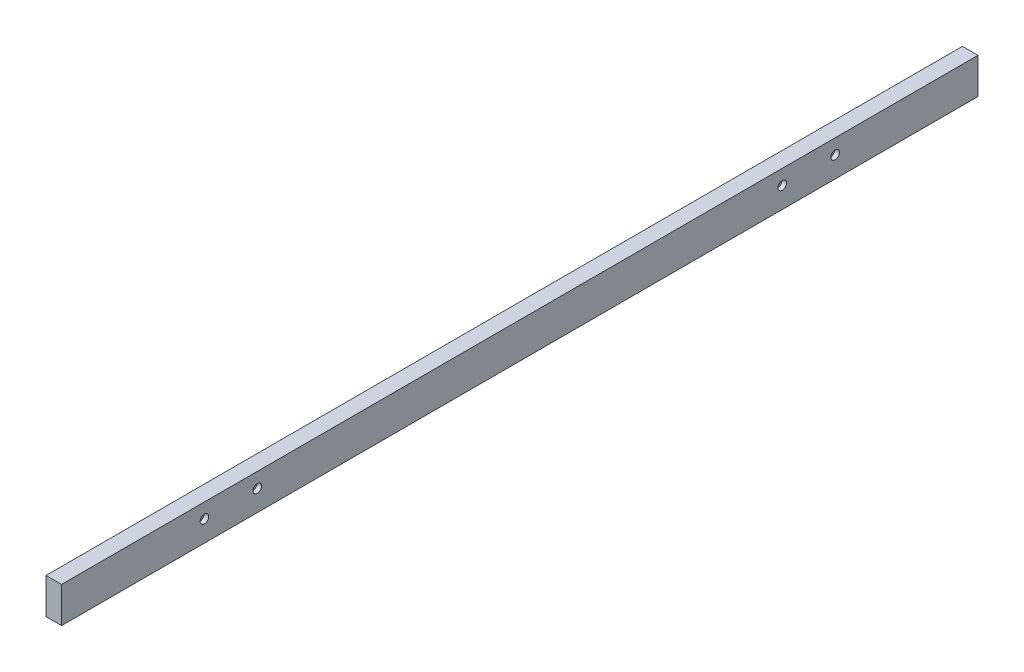
from build123d import *

# Parameters (mm, degrees)
SKETCH1_W                                    = 10
SKETCH1_H                                    = 590
BOSS_EXTRUDE1_DEPTH                          = 23
CBORE_FOR_M2_5_HEX_SOCKET_HEAD_CAP_S_2_COUNT = 2
CBORE_FOR_M2_5_HEX_SOCKET_HEAD_CAP_S_2_PITCH = 34
CUT_EXTRUDE1_START                           = -1
SKETCH10_W                                   = 5
SKETCH10_H                                   = 42
CUT_EXTRUDE1_DEPTH                           = 17
CBORE_FOR_M2_HEX_SOCKET_HEAD_CAP_SCR_3_COUNT = 2
CBORE_FOR_M2_HEX_SOCKET_HEAD_CAP_SCR_3_PITCH = 26


with BuildPart() as part:
    # Sketch1 → Boss-Extrude1 (new body)
    with BuildSketch(Plane(origin=(0, 0, 0), x_dir=(1, 0, 0), z_dir=(0, 1, 0))):
        Rectangle(SKETCH1_W, SKETCH1_H)
    extrude(amount=BOSS_EXTRUDE1_DEPTH)

    # Sketch9 → CBORE for M2.5 Hex Socket Head Cap Screw1 (revolve, cut)
    with BuildSketch(Plane(origin=(5, 13.5, 203), x_dir=(0, 0, -1), z_dir=(0, 1, 0))):
        Polygon((0, 0), (0, 22.811247898), (1.45, 21.94), (1.45, 2.9), (2.75, 2.9), (2.75, 0), align=None)
    cbore_for_m2_5_hex_socket_head_cap_screw = revolve(axis=Axis((11.35, 13.5, 203), (-1, 0, 0)), mode=Mode.SUBTRACT)

    # CBORE for M2.5 Hex Socket Head Cap S 2: CBORE for M2.5 Hex Socket Head Cap Screw1 ×2
    with Locations(*[(0, 0, -i * CBORE_FOR_M2_5_HEX_SOCKET_HEAD_CAP_S_2_PITCH) for i in range(1, CBORE_FOR_M2_5_HEX_SOCKET_HEAD_CAP_S_2_COUNT)]):
        add(cbore_for_m2_5_hex_socket_head_cap_screw, mode=Mode.SUBTRACT)

    # Mirror1: CBORE for M2.5 Hex Socket Head Cap Screw1 across plane
    add(cbore_for_m2_5_hex_socket_head_cap_screw.mirror(Plane.XY), mode=Mode.SUBTRACT)

    # Mirror1 copy 1 sketch → Mirror1 copy 1 (revolve, cut)
    with BuildSketch(Plane(origin=(5, 13.5, -169), x_dir=(0, 0, 1), z_dir=(0, 1, 0))):
        Polygon((0, 0), (0, -22.811247898), (1.45, -21.94), (1.45, -2.9), (2.75, -2.9), (2.75, 0), align=None)
    revolve(axis=Axis((11.35, 13.5, -169), (1, 0, 0)), mode=Mode.SUBTRACT)

    # Sketch10 → Cut-Extrude1 (cut)
    with BuildSketch(Plane(origin=(0, 23, 0), x_dir=(1, 0, 0), z_dir=(0, 1, 0)).offset(CUT_EXTRUDE1_START)):
        with Locations((-2.5, 186)):
            Rectangle(SKETCH10_W, SKETCH10_H)
    cut_extrude1 = extrude(amount=-CUT_EXTRUDE1_DEPTH, mode=Mode.SUBTRACT)

    # Mirror2: Cut-Extrude1 across plane
    add(cut_extrude1.mirror(Plane.XY), mode=Mode.SUBTRACT)

    # Sketch12 → CBORE for M2 Hex Socket Head Cap Screw1 (revolve, cut)
    with BuildSketch(Plane(origin=(-2.5, 0, -173), x_dir=(0, 0, -1), z_dir=(1, 0, 0))):
        Polygon((0, 0), (0, 20.721032743), (1.2, 20), (1.2, 2.4), (2.2, 2.4), (2.2, 0), align=None)
    cbore_for_m2_hex_socket_head_cap_screw1 = revolve(axis=Axis((-2.5, -6.35, -173), (0, 1, 0)), mode=Mode.SUBTRACT)

    # CBORE for M2 Hex Socket Head Cap Scr 3: CBORE for M2 Hex Socket Head Cap Screw1 ×2
    with Locations(*[(0, 0, -i * CBORE_FOR_M2_HEX_SOCKET_HEAD_CAP_SCR_3_PITCH) for i in range(1, CBORE_FOR_M2_HEX_SOCKET_HEAD_CAP_SCR_3_COUNT)]):
        add(cbore_for_m2_hex_socket_head_cap_screw1, mode=Mode.SUBTRACT)


solid = part.part
